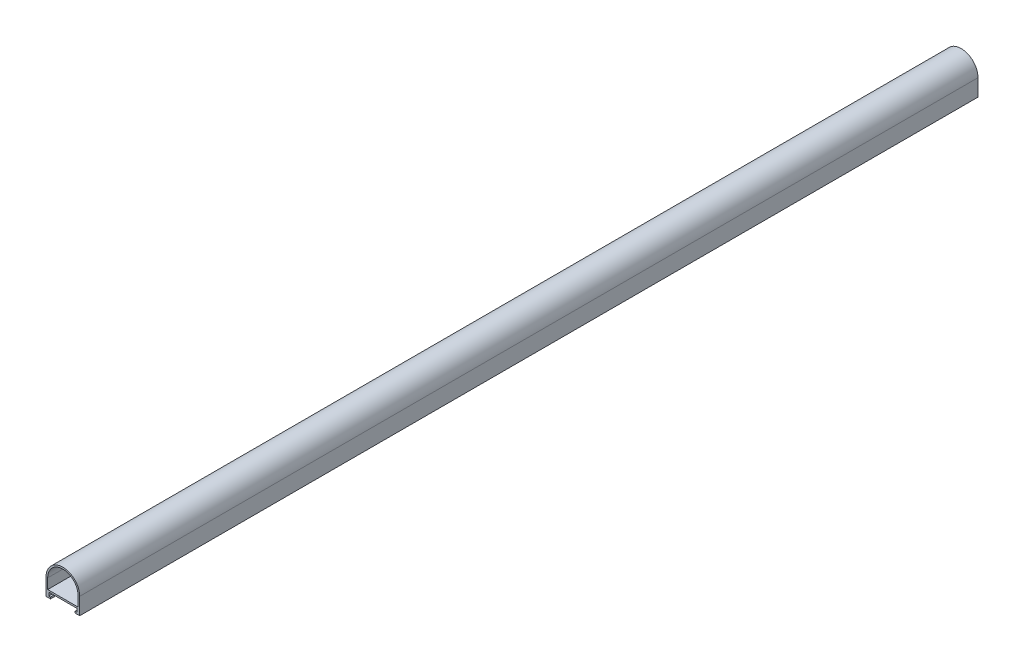
from build123d import *

# Parameters (mm, degrees)
BOSS_EXTRUDE1_DEPTH = 800
CUT_EXTRUDE1_DEPTH  = 800
CUT_EXTRUDE2_DEPTH  = 803.081458262


with BuildPart() as part:
    # Sketch1 → Boss-Extrude1 (new body)
    with BuildSketch(Plane.XY):
        with BuildLine():
            Line((-25.764376508, 0), (-25.764376508, -15))
            Line((-25.764376508, -15), (-55.764376508, -15))
            Line((-55.764376508, -15), (-55.764376508, 0))
            ThreePointArc((-55.764376508, 0), (-40.764376508, 15), (-25.764376508, 0))
        make_face()
    extrude(amount=BOSS_EXTRUDE1_DEPTH)

    # Sketch2 → Cut-Extrude1 (cut)
    with BuildSketch(Plane.XY.offset(800)):
        with BuildLine():
            Line((-27.264376508, 0), (-27.264376508, -9))
            Line((-27.264376508, -9), (-54.264376508, -9))
            Line((-54.264376508, -9), (-54.264376508, 0))
            ThreePointArc((-54.264376508, 0), (-40.764376508, 13.5), (-27.264376508, 0))
        make_face()
    extrude(amount=-CUT_EXTRUDE1_DEPTH, mode=Mode.SUBTRACT)

    # Sketch3 → Cut-Extrude2 (cut, through all)
    with BuildSketch(Plane.XY.offset(800)):
        Polygon((-51.764376508, -15), (-51.764376508, -13.5), (-53.264376508, -13.5), (-53.264376508, -10.5), (-28.264376508, -10.5), (-28.264376508, -13.5), (-29.764376508, -13.5), (-29.764376508, -15), align=None)
    extrude(amount=-CUT_EXTRUDE2_DEPTH, mode=Mode.SUBTRACT)


solid = part.part
